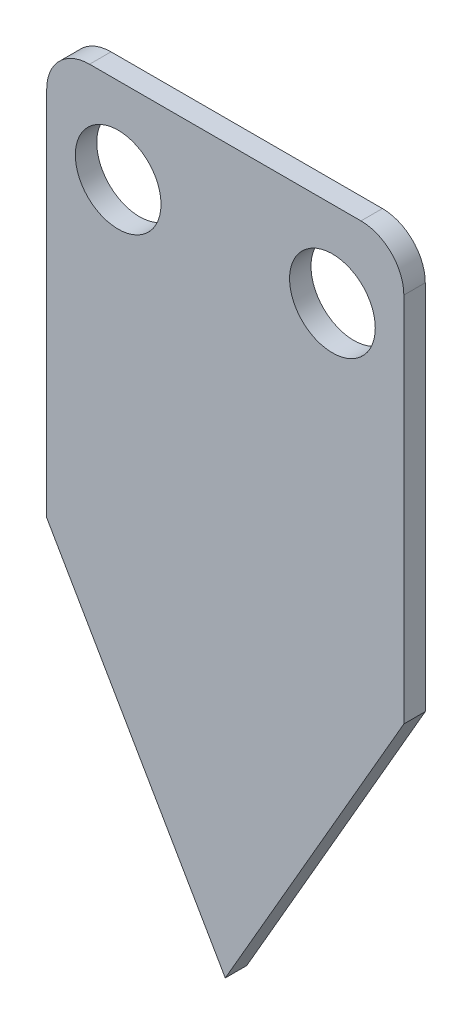
SolidWorks part; units mm, degrees
ref_plane "前视基准面" through (0, 0, 0) normal (0, 0, 1) x (1, 0, 0)
ref_plane "上视基准面" through (0, 0, 0) normal (0, 1, 0) x (1, 0, 0)
ref_plane "右视基准面" through (0, 0, 0) normal (1, 0, 0) x (0, 0, -1)
sketch "草图1" plane through (0, 0, 0) normal (0, 0, 1) x (1, 0, 0)
  line L0 (-12.5, 0) -> (12.5, 0)
  line L1 (12.5, 0) -> (12.5, -29)
  line L2 (-12.5, -29) -> (0, -50.6506)
  line L3 (0, -50.6506) -> (12.5, -29)
  line L6 (-12.5, -29) -> (-12.5, 0)
  line L7 (0, 0) -> (0, -88.4502) construction
  dimension "D1" = 25
  dimension "D2" = 29
  dimension "D3" = 150
extrude "凸台-拉伸1" add sketch "草图1" along normal blind 1.5
hole_wizard "Ø6.0 (6) 直径孔1" positions "草图3" profile "草图2" hole size "Ø6.0" standard "GB" end condition through all
sketch "草图3" plane through (0, 0, 1.5) normal (0, 0, 1) x (1, 0, 0)
  line L0 (0, 0) -> (0, -28.6169) construction
  line L2 (12.5, 0) -> (-12.5, 0) construction
  point P0 (-7.5, -6)
  point P2 (7.5, -6)
  dimension "D1" = 15
  dimension "D2" = 6
sketch "草图2" plane through (-7.5, -6, 1.5) normal (1, 0, 0) x (0, -1, 0)
  line L0 (0, 0) -> (0, 1.5)
  line L1 (0, 1.5) -> (3, 1.5)
  line L2 (3, 1.5) -> (3, 0)
  line L5 (3, 0) -> (0, 0)
  line L11 (0, -6.35) -> (0, 107.95) construction
  dimension "通孔孔直径" = 6
  dimension "通孔孔深度" = 1.5
fillet "圆角1" radius 3 2 edges at (12.5, 0, 0.75) (-12.5, 0, 0.75)
